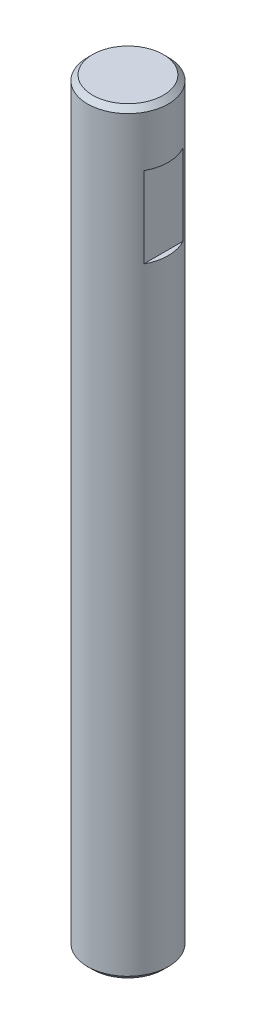
from build123d import *

# Parameters (mm, degrees)
SKETCH1_R           = 4
BOSS_EXTRUDE1_DEPTH = 75
CHAMFER1_SIZE       = 0.5
SKETCH2_W           = 1
SKETCH2_H           = 8
CUT_EXTRUDE1_DEPTH  = 5


with BuildPart() as part:
    # Sketch1 → Boss-Extrude1 (new body)
    with BuildSketch(Plane(origin=(0, 0, 0), x_dir=(1, 0, 0), z_dir=(0, 1, 0))):
        with Locations(Location((0, 0, 0), (0, 0, 270))):
            Circle(SKETCH1_R)
    extrude(amount=BOSS_EXTRUDE1_DEPTH)

    # Chamfer1
    chamfer1_edges = [part.edges().sort_by_distance(p)[0] for p in [
        (0, 0, -4),
        (0, 75, -4),
    ]]
    chamfer(chamfer1_edges, length=CHAMFER1_SIZE)

    # Sketch2 → Cut-Extrude1 (cut, symmetric)
    with BuildSketch(Plane.XY):
        with Locations((4, 65.5)):
            Rectangle(SKETCH2_W, SKETCH2_H)
    extrude(amount=CUT_EXTRUDE1_DEPTH, both=True, mode=Mode.SUBTRACT)


solid = part.part
